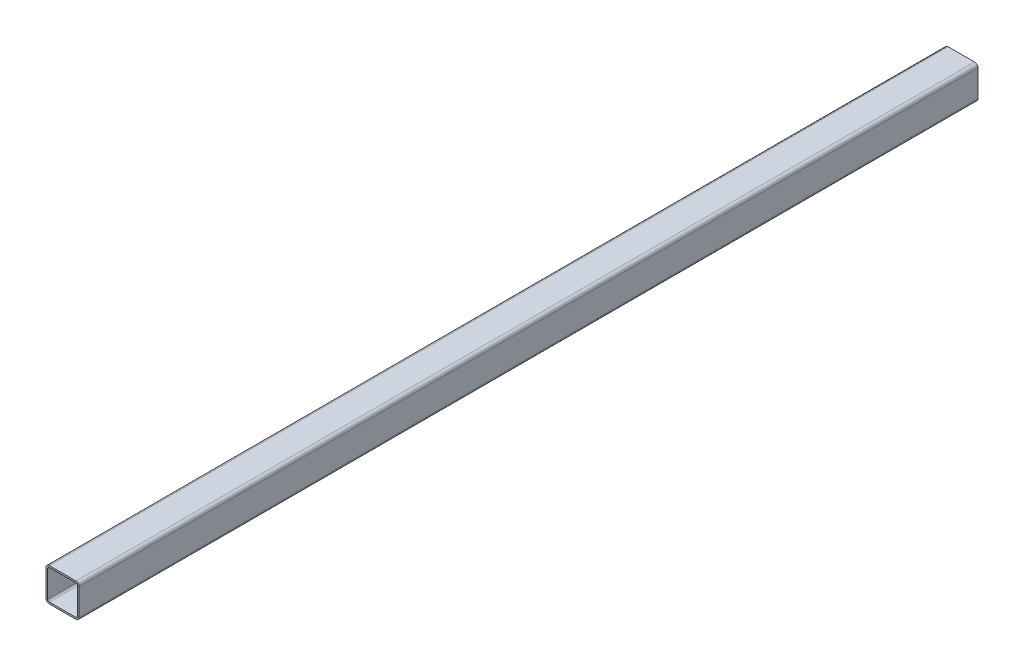
from build123d import *

# Parameters (mm, degrees)
SKETCH1_W           = 40
SKETCH1_H           = 40
SKETCH1_W_2         = 36
SKETCH1_H_2         = 36
BOSS_EXTRUDE1_DEPTH = 1082
FILLET1_R           = 2
FILLET2_R           = 4


with BuildPart() as part:
    # Sketch1 → Boss-Extrude1 (new body)
    with BuildSketch(Plane.XY):
        Rectangle(SKETCH1_W, SKETCH1_H)
        Rectangle(SKETCH1_W_2, SKETCH1_H_2, mode=Mode.SUBTRACT)
    extrude(amount=BOSS_EXTRUDE1_DEPTH)

    # Fillet1
    fillet1_edges = [part.edges().sort_by_distance(p)[0] for p in [
        (18, -18, 541),
        (18, 18, 541),
        (-18, 18, 541),
        (-18, -18, 541),
    ]]
    fillet(fillet1_edges, radius=FILLET1_R)

    # Fillet2
    fillet2_edges = [part.edges().sort_by_distance(p)[0] for p in [
        (20, -20, 541),
        (-20, -20, 541),
        (-20, 20, 541),
        (20, 20, 541),
    ]]
    fillet(fillet2_edges, radius=FILLET2_R)


solid = part.part
